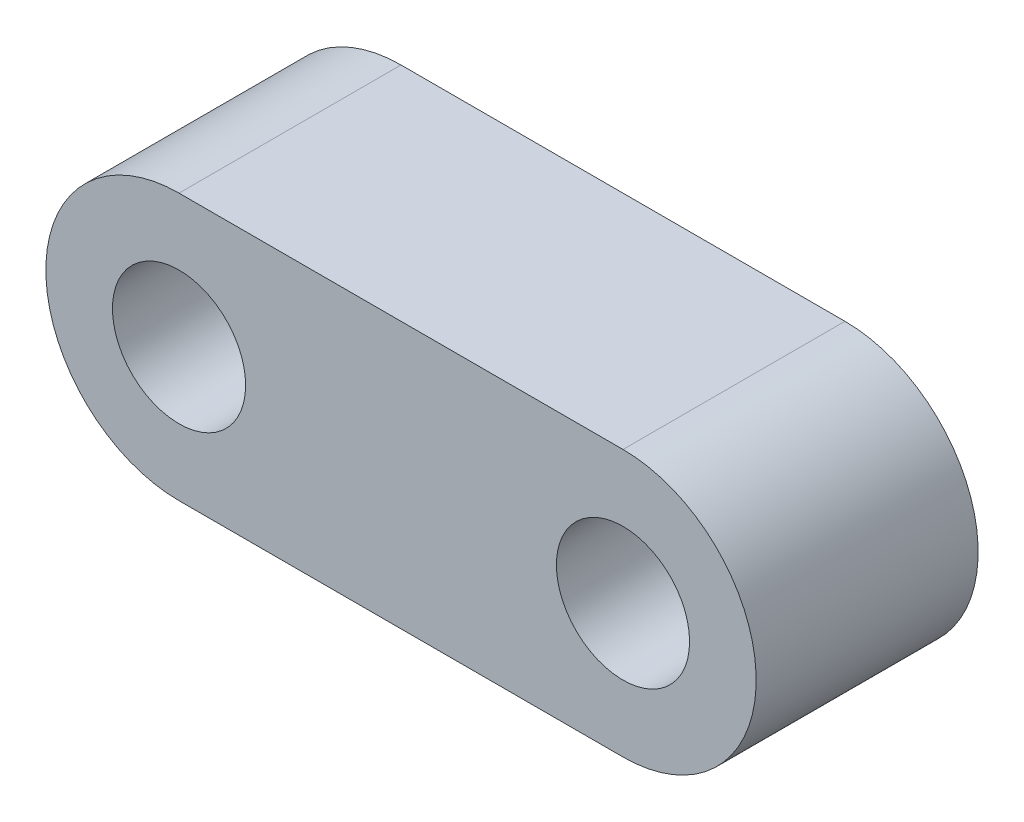
SolidWorks part; units mm, degrees
ref_plane "Front Plane" through (0, 0, 0) normal (0, 0, 1) x (1, 0, 0)
ref_plane "Top Plane" through (0, 0, 0) normal (0, 1, 0) x (1, 0, 0)
ref_plane "Right Plane" through (0, 0, 0) normal (1, 0, 0) x (0, 0, -1)
sketch "Sketch1" plane through (0, 0, 0) normal (0, 0, 1) x (1, 0, 0)
  line L0 (0, -6) -> (20, -6)
  line L1 (0, 6) -> (20, 6)
  line L2 (0, 0) -> (20, 0) construction
  circle A0 centre (0, 0) radius 3
  arc A1 (0, 6) -> (0, -6) centre (0, 0) ccw
  circle A2 centre (20, 0) radius 3
  arc A3 (20, -6) -> (20, 6) centre (20, 0) ccw
  dimension "D1" = 20
  dimension "D2" = 6
  dimension "D3" = 6
  dimension "D4" = 12
  dimension "D5" = 12
  dimension "D6" = 12
  dimension "D7" = 6
extrude "Boss-Extrude1" add sketch "Sketch1" along normal blind 10
